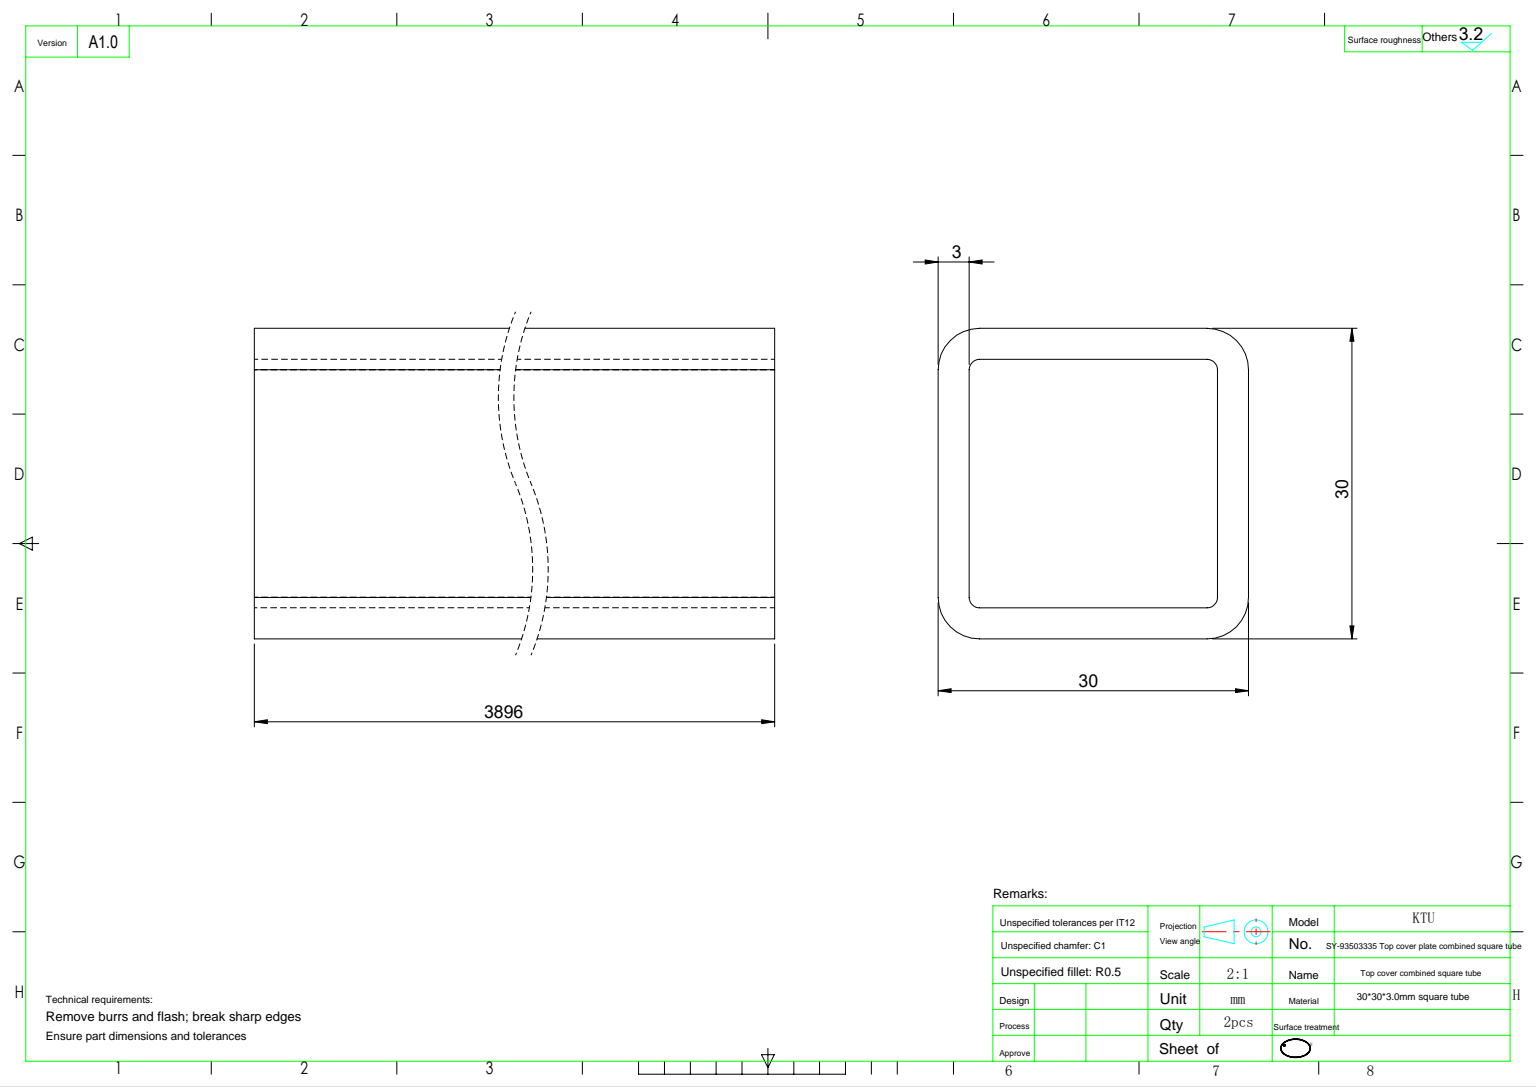
SolidWorks part; units mm, degrees
ref_plane "前视基准面" through (0, 0, 0) normal (0, 0, 1) x (1, 0, 0)
ref_plane "上视基准面" through (0, 0, 0) normal (0, 1, 0) x (1, 0, 0)
ref_plane "右视基准面" through (0, 0, 0) normal (1, 0, 0) x (0, 0, -1)
sketch "草图2" plane through (0, 0, 0) normal (0, 0, 1) x (1, 0, 0)
  line L1 (-11, 15) -> (11, 15)
  line L2 (-15, 11) -> (-15, -11)
  line L3 (-11, -15) -> (11, -15)
  line L4 (15, 11) -> (15, -11)
  line L5 (-15, 15) -> (15, -15) construction
  line L6 (-15, -15) -> (15, 15) construction
  arc A0 (11, 15) -> (15, 11) centre (11, 11) cw
  arc A1 (11, -15) -> (15, -11) centre (11, -11) ccw
  arc A2 (-15, -11) -> (-11, -15) centre (-11, -11) ccw
  arc A3 (-11, 15) -> (-15, 11) centre (-11, 11) ccw
  point P0 (0, 0)
  dimension "D3" = 4
  dimension "D1" = 30
  dimension "D2" = 30
extrude "拉伸-薄壁1" add sketch "草图2" along normal mid plane 3896 thin
